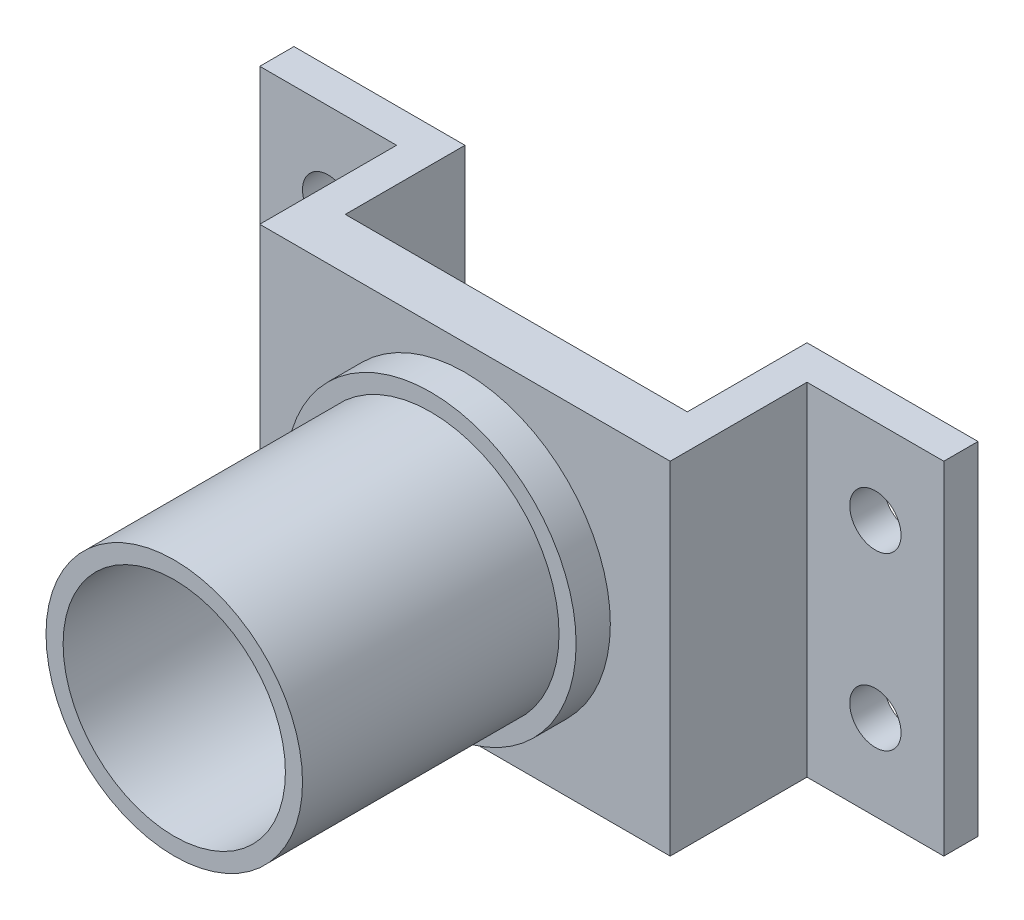
from build123d import *

# Parameters (mm, degrees)
SKETCH1_R           = 7.5
SKETCH1_R_2         = 6.5
BOSS_EXTRUDE1_DEPTH = 22
BOSS_EXTRUDE2_START = 2
SKETCH2_R           = 8.5
SKETCH2_R_2         = 7.5
BOSS_EXTRUDE2_DEPTH = 2
BOSS_EXTRUDE4_START = 2
SKETCH5_R           = 7.5
SKETCH5_R_2         = 6.5
BOSS_EXTRUDE4_DEPTH = 2
BOSS_EXTRUDE5_START = 2
SKETCH6_R           = 8.5
SKETCH6_R_2         = 6.5
BOSS_EXTRUDE5_DEPTH = 2
SKETCH7_W           = 30
SKETCH7_H           = 20
BOSS_EXTRUDE6_DEPTH = 10
SKETCH8_W           = 20
SKETCH8_H           = 7
CUT_EXTRUDE1_DEPTH  = 34.301651611
SKETCH9_W           = 5
SKETCH9_H           = 20
BOSS_EXTRUDE7_DEPTH = 2
SKETCH12_R          = 6.5
CUT_EXTRUDE3_DEPTH  = 31
SKETCH13_W          = 3
SKETCH13_H          = 20
CUT_EXTRUDE4_DEPTH  = 8
SKETCH11_R          = 1.5
CUT_EXTRUDE2_DEPTH  = 34.541019662


with BuildPart() as part:
    # Sketch1 → Boss-Extrude1 (new body)
    with BuildSketch(Plane.XY):
        Circle(SKETCH1_R)
        Circle(SKETCH1_R_2, mode=Mode.SUBTRACT)
    extrude(amount=BOSS_EXTRUDE1_DEPTH)

    # Sketch2 → Boss-Extrude2 (add)
    with BuildSketch(Plane(origin=(0, 0, 7), x_dir=(-1, 0, 0), z_dir=(0, 0, -1)).offset(BOSS_EXTRUDE2_START)):
        Circle(SKETCH2_R)
        Circle(SKETCH2_R_2, mode=Mode.SUBTRACT)
    extrude(amount=-BOSS_EXTRUDE2_DEPTH)

    # Sketch5 → Boss-Extrude4 (add)
    with BuildSketch(Plane(origin=(0, 0, 0), x_dir=(-1, 0, 0), z_dir=(0, 0, -1)).offset(BOSS_EXTRUDE4_START)):
        Circle(SKETCH5_R)
        Circle(SKETCH5_R_2, mode=Mode.SUBTRACT)
    extrude(amount=-BOSS_EXTRUDE4_DEPTH)

    # Sketch6 → Boss-Extrude5 (add)
    with BuildSketch(Plane(origin=(0, 0, -2), x_dir=(-1, 0, 0), z_dir=(0, 0, -1)).offset(BOSS_EXTRUDE5_START)):
        Circle(SKETCH6_R)
        Circle(SKETCH6_R_2, mode=Mode.SUBTRACT)
    extrude(amount=-BOSS_EXTRUDE5_DEPTH)

    # Sketch7 → Boss-Extrude6 (add)
    with BuildSketch(Plane(origin=(0, 0, 5), x_dir=(-1, 0, 0), z_dir=(0, 0, -1))):
        Rectangle(SKETCH7_W, SKETCH7_H)
    extrude(amount=BOSS_EXTRUDE6_DEPTH)

    # Sketch8 → Cut-Extrude1 (cut, through all)
    with BuildSketch(Plane.XZ.offset(10)):
        with Locations((0, -1.5)):
            Rectangle(SKETCH8_W, SKETCH8_H)
    extrude(amount=-CUT_EXTRUDE1_DEPTH, mode=Mode.SUBTRACT)

    # Sketch9 → Boss-Extrude7 (add)
    with BuildSketch(Plane(origin=(0, 0, -5), x_dir=(-1, 0, 0), z_dir=(0, 0, -1))):
        with Locations((-17.5, 0)):
            Rectangle(SKETCH9_W, SKETCH9_H)
        with Locations((17.5, 0)):
            Rectangle(SKETCH9_W, SKETCH9_H)
    extrude(amount=-BOSS_EXTRUDE7_DEPTH)

    # Sketch12 → Cut-Extrude3 (cut, through all)
    with BuildSketch(Plane(origin=(0, 0, 2), x_dir=(-1, 0, 0), z_dir=(0, 0, -1))):
        Circle(SKETCH12_R)
    extrude(amount=-CUT_EXTRUDE3_DEPTH, mode=Mode.SUBTRACT)

    # Sketch13 → Cut-Extrude4 (cut)
    with BuildSketch(Plane.XY.offset(5)):
        with Locations((-13.5, 0)):
            Rectangle(SKETCH13_W, SKETCH13_H)
        with Locations((13.5, 0)):
            Rectangle(SKETCH13_W, SKETCH13_H)
    extrude(amount=-CUT_EXTRUDE4_DEPTH, mode=Mode.SUBTRACT)

    # Sketch11 → Cut-Extrude2 (cut, through all)
    with BuildSketch(Plane.XY.offset(-3)):
        with Locations((16, 5)):
            Circle(SKETCH11_R)
        with Locations((16, -5)):
            Circle(SKETCH11_R)
        with Locations(Location((-16, -5, 0), (0, 0, 180))):
            Circle(SKETCH11_R)
        with Locations(Location((-16, 5, 0), (0, 0, 180))):
            Circle(SKETCH11_R)
    extrude(amount=-CUT_EXTRUDE2_DEPTH, mode=Mode.SUBTRACT)


solid = part.part
